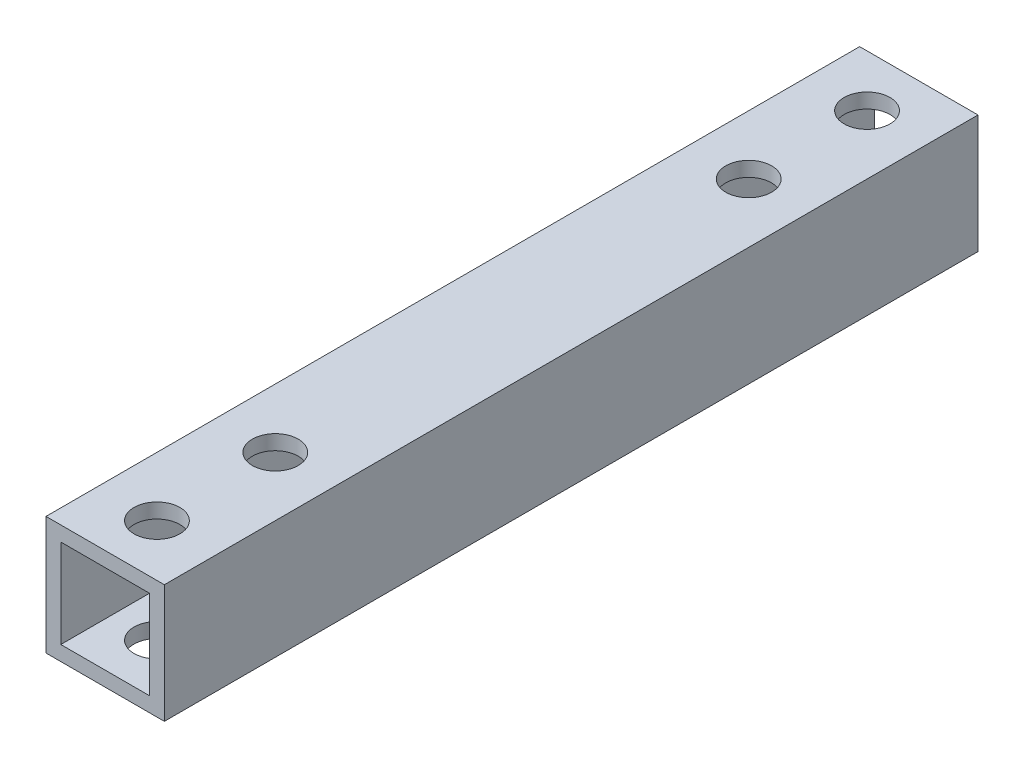
from build123d import *

# Parameters (mm, degrees)
SKETCH_1_W          = 8
SKETCH_1_H          = 8
SKETCH_1_W_2        = 6
SKETCH_1_H_2        = 6
EXTRUDE_1_DEPTH     = 55
SKETCH_3_R          = 1.55
CUT_EXTRUDE_1_DEPTH = 55


with BuildPart() as part:
    # 草图1 → 凸台-拉伸1 (new body)
    with BuildSketch(Plane.XY):
        Rectangle(SKETCH_1_W, SKETCH_1_H)
        Rectangle(SKETCH_1_W_2, SKETCH_1_H_2, mode=Mode.SUBTRACT)
    extrude(amount=-EXTRUDE_1_DEPTH)

    # 草图3 → 切除-拉伸1 (cut)
    with BuildSketch(Plane(origin=(0, 4, 0), x_dir=(1, 0, 0), z_dir=(0, 1, 0))):
        with Locations(Location((0, 3.5, 0), (0, 0, 90))):
            Circle(SKETCH_3_R)
        with Locations(Location((0, 11.5, 0), (0, 0, 90))):
            Circle(SKETCH_3_R)
        with Locations(Location((0, 43.5, 0), (0, 0, 90))):
            Circle(SKETCH_3_R)
        with Locations(Location((0, 51.5, 0), (0, 0, 90))):
            Circle(SKETCH_3_R)
    extrude(amount=-CUT_EXTRUDE_1_DEPTH, mode=Mode.SUBTRACT)


solid = part.part
